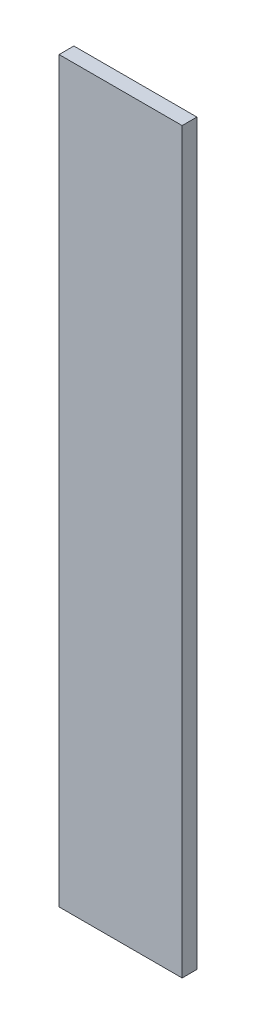
SolidWorks part; units mm, degrees
ref_plane "前视基准面" through (0, 0, 0) normal (0, 0, 1) x (1, 0, 0)
ref_plane "上视基准面" through (0, 0, 0) normal (0, 1, 0) x (1, 0, 0)
ref_plane "右视基准面" through (0, 0, 0) normal (1, 0, 0) x (0, 0, -1)
other "Configuration Table"
sketch "草图1" plane through (0, 0, 0) normal (0, 0, 1) x (1, 0, 0)
  line L0 (-12.5, -75) -> (12.5, -75)
  line L1 (12.5, -75) -> (12.5, 75)
  line L2 (12.5, 75) -> (-12.5, 75)
  line L3 (-12.5, 75) -> (-12.5, -75)
  point P0 (0, 0)
  dimension "D1" = 12.5
  dimension "D2" = 25
  dimension "D3" = 75
  dimension "D4" = 150
extrude "凸台-拉伸1" add sketch "草图1" against normal mid plane 3
